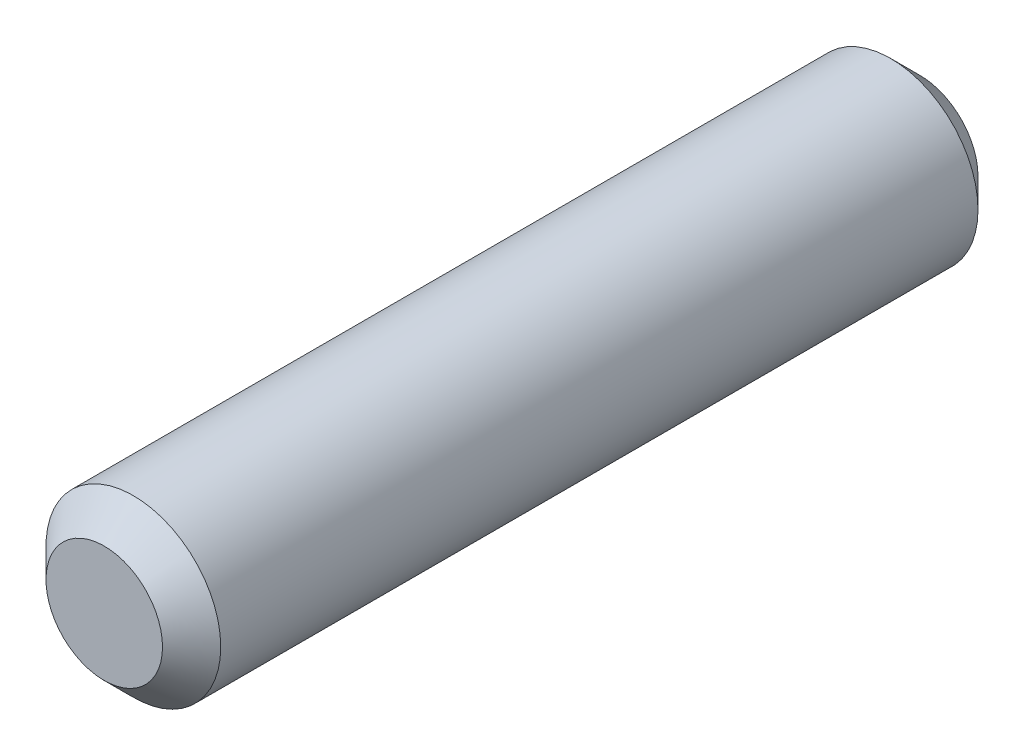
SolidWorks part; units mm, degrees
ref_plane "Front Plane" through (0, 0, 0) normal (0, 0, 1) x (1, 0, 0)
ref_plane "Top Plane" through (0, 0, 0) normal (0, 1, 0) x (1, 0, 0)
ref_plane "Right Plane" through (0, 0, 0) normal (1, 0, 0) x (0, 0, -1)
other "Configuration Table"
sketch "Sketch1" plane through (0, 0, 0) normal (0, 0, 1) x (1, 0, 0)
  circle A0 centre (0, 0) radius 1.5
  dimension "D1" = 3
extrude "Boss-Extrude1" add sketch "Sketch1" along normal blind 14
chamfer "Chamfer1" distance 0.5 angle 45 2 edges at (1.5, 0, 0) (1.5, 0, 14)
